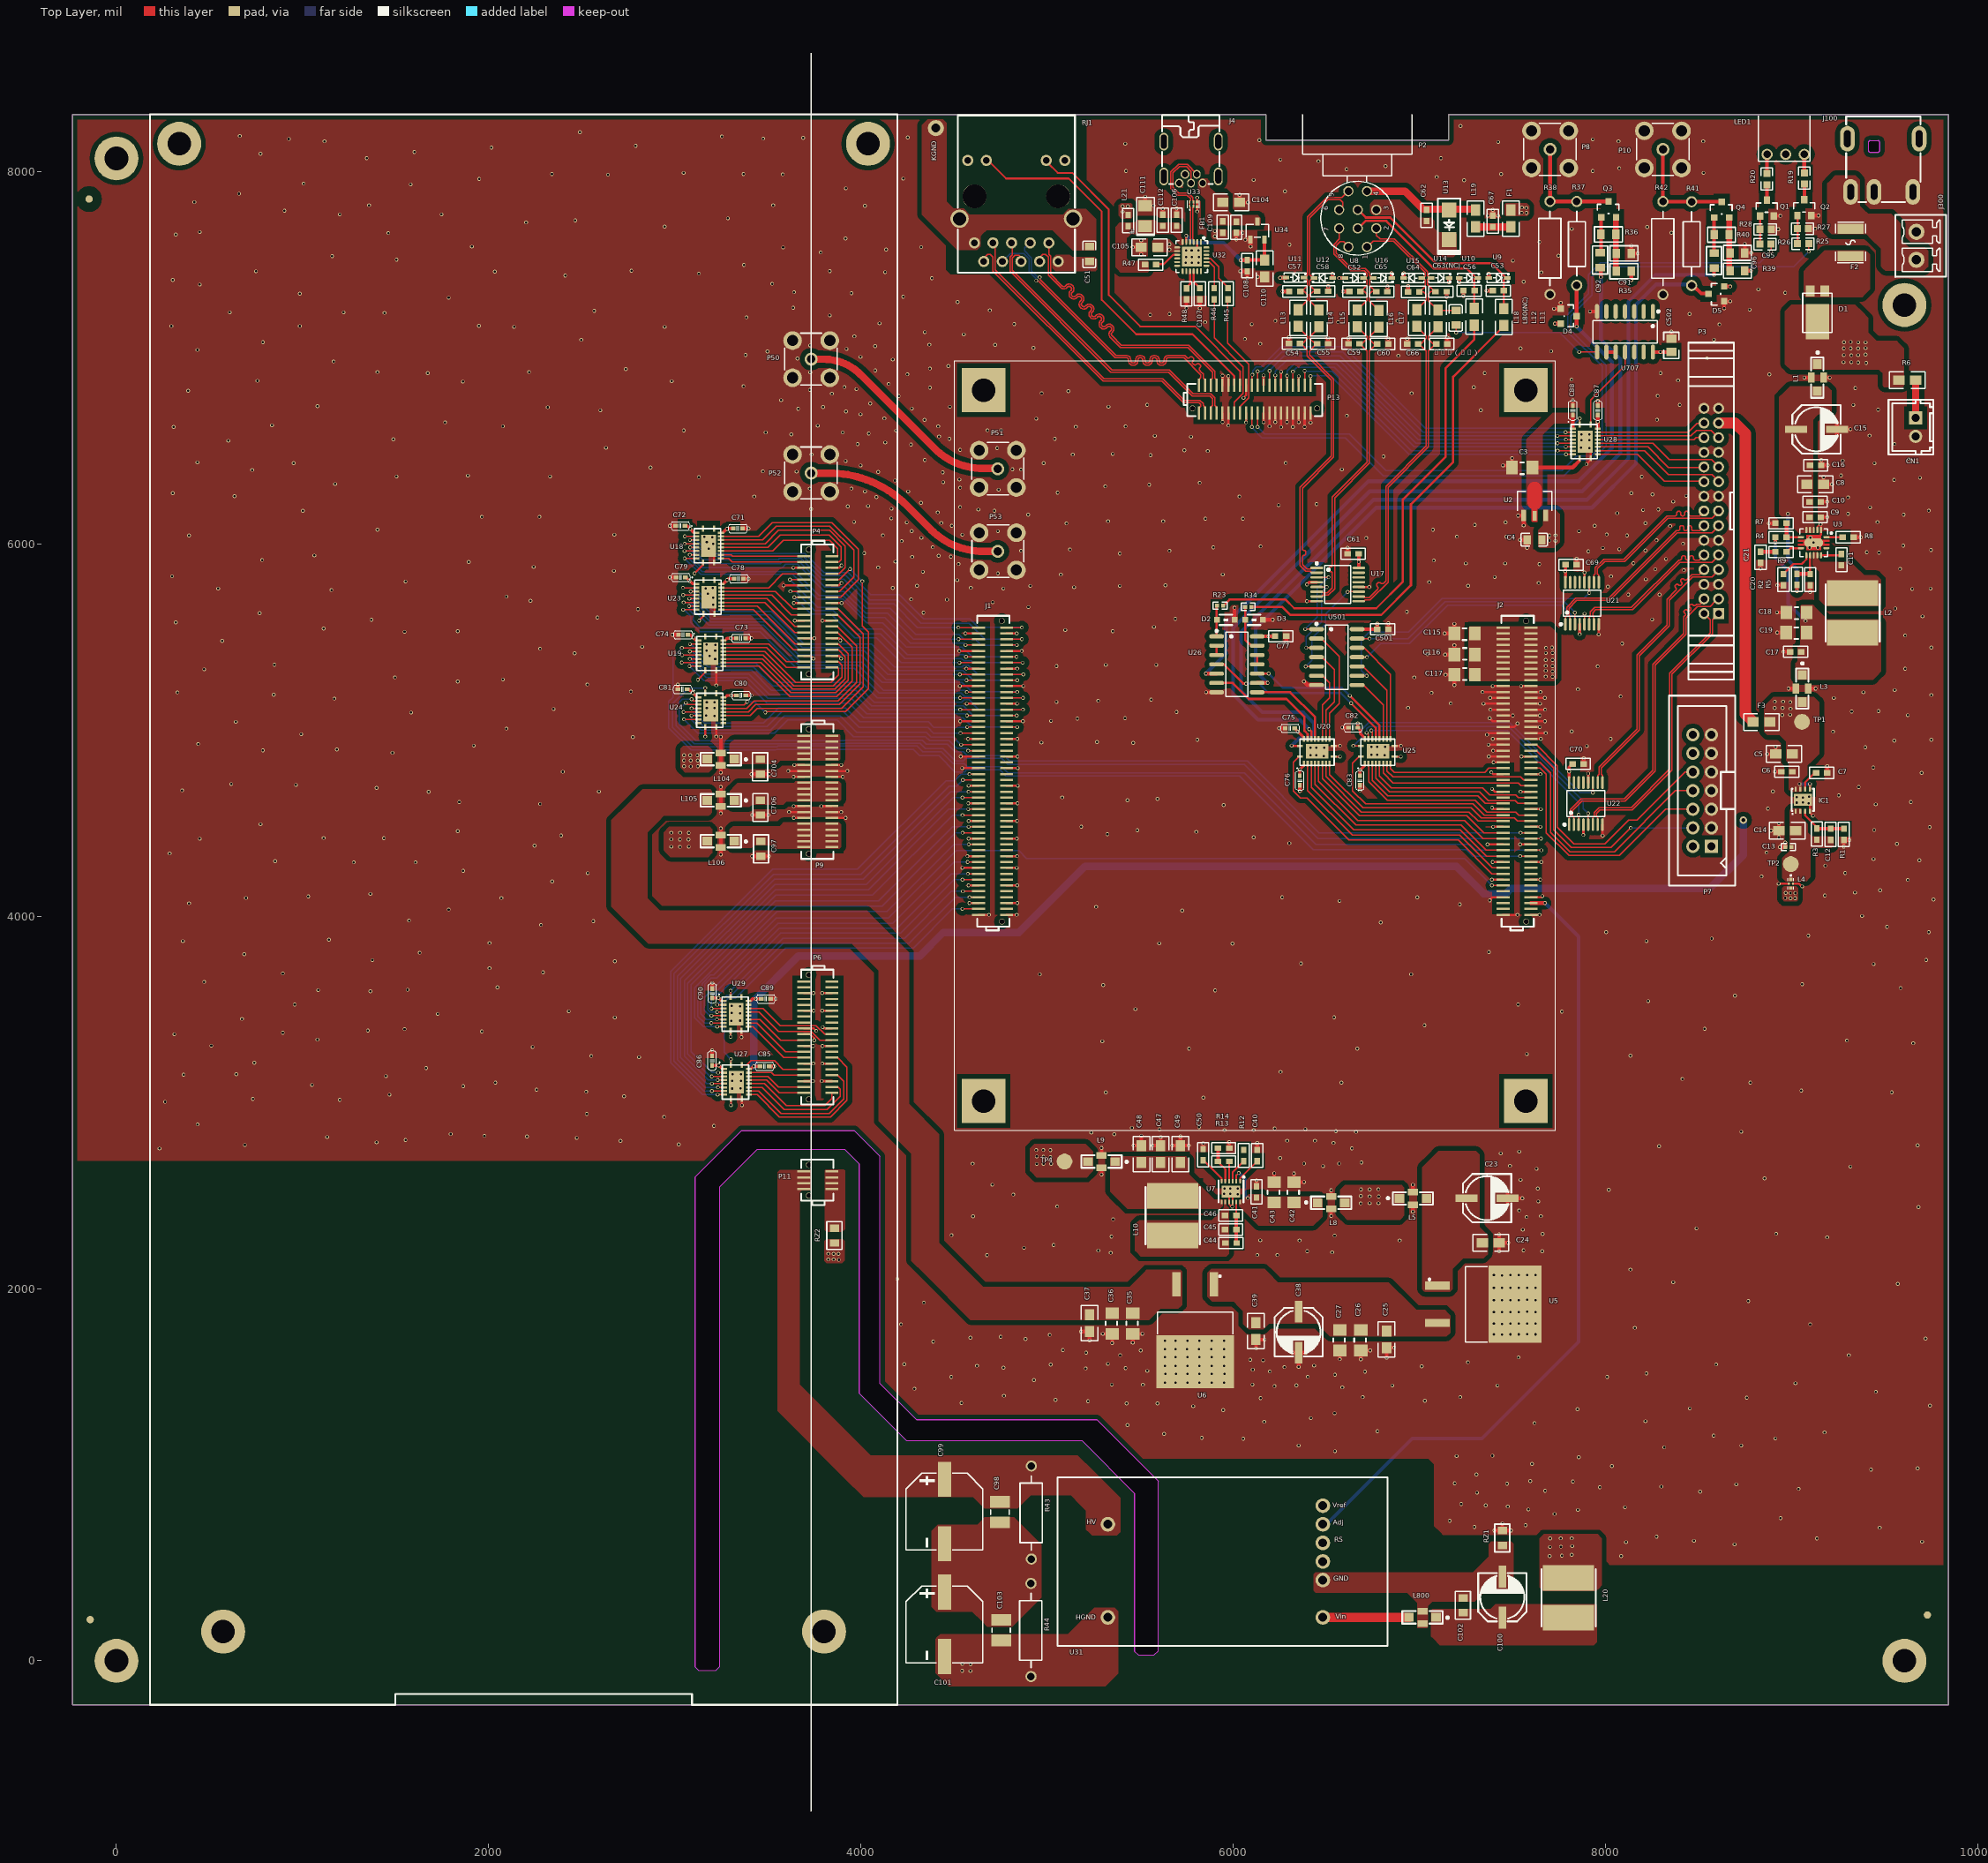
[diagram p0: Top Layer view]
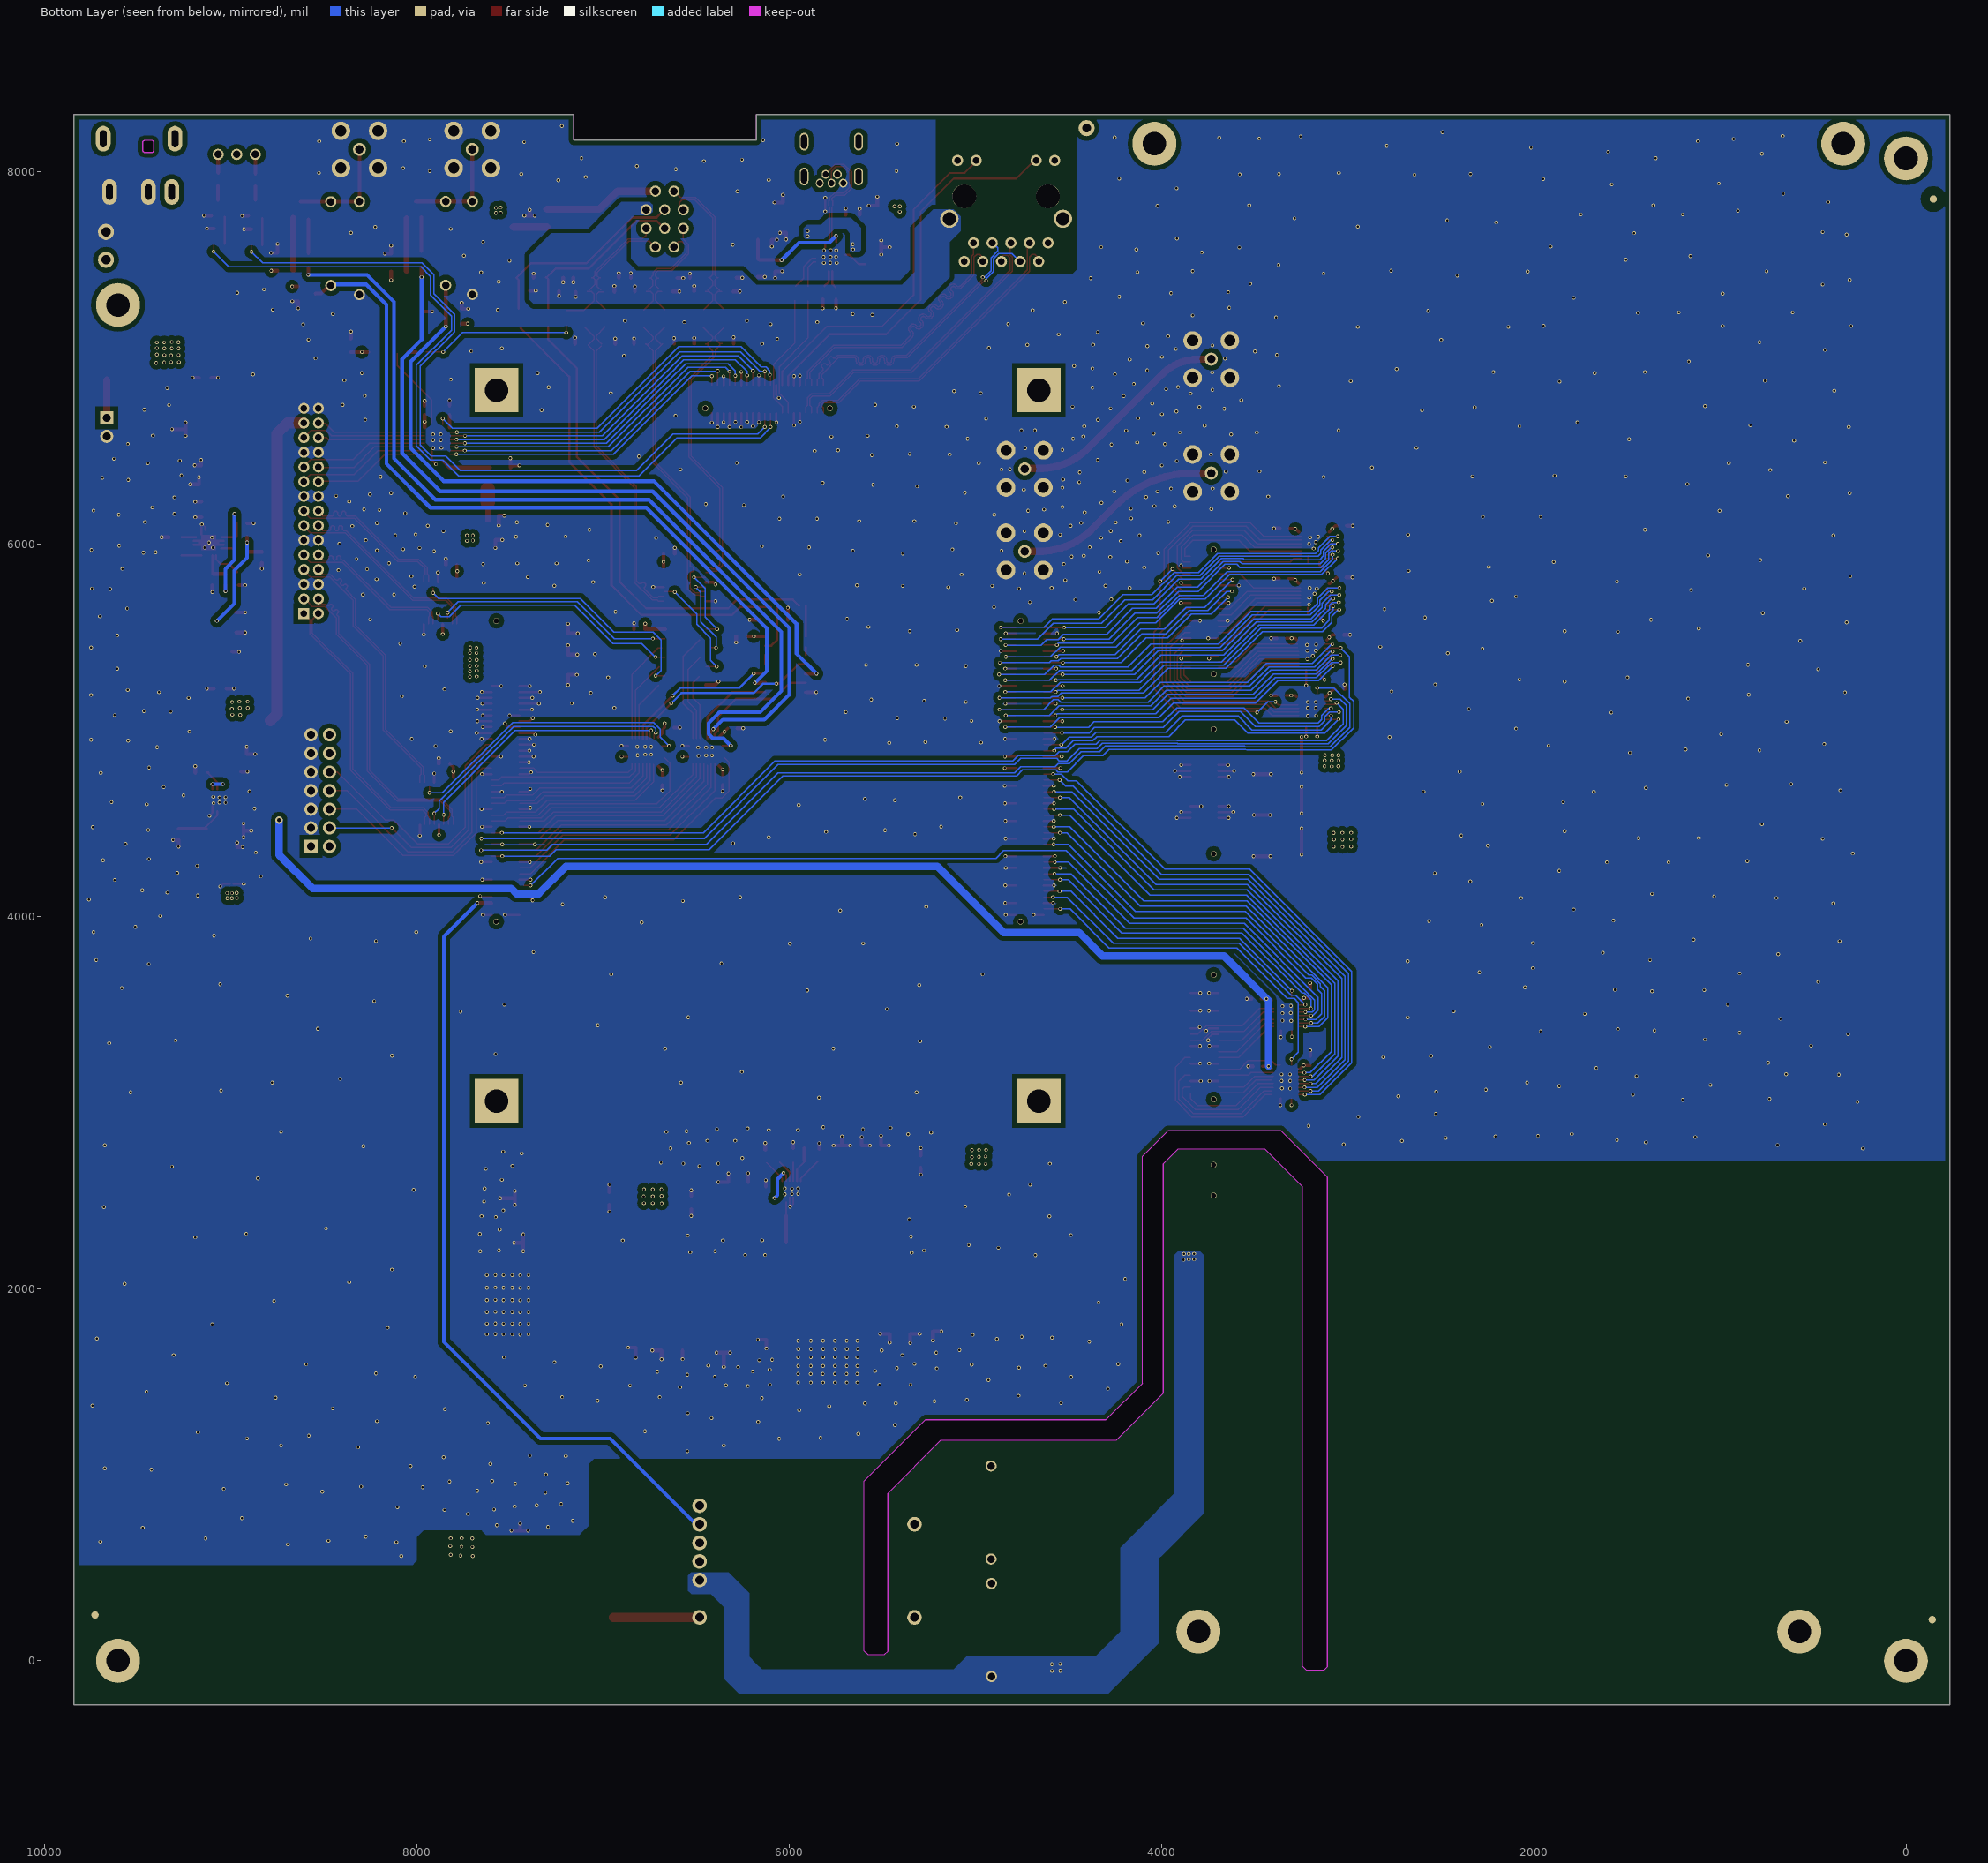
[diagram p1: Bottom Layer view, seen from below]
# Altium PCB MISC82191.PcbDoc (part 1 of 9)
Units mil, origin at the board's own origin, x right, y up, seen from the top; angles counter-clockwise.
Board outline 10078.74 x 8543.31 mil, 4 copper layers (Top Layer, GND, POWER, Bottom Layer); 238 components, 299 nets, 1297 pads, 1665 vias.

## Layer stack, top to bottom (the 12.6 mil dielectric is the usual default, probably not edited)
Top Layer: signal copper 1.4
Dielectric: core 12.6, FR-4, Dk 4.8
GND: plane copper 1.4, net GND
Dielectric: prepreg 12.6, FR-4, Dk 4.8
POWER: plane copper 1.4, net (Multiple Nets)
Dielectric: core 12.6, FR-4, Dk 4.8
Bottom Layer: signal copper 1.4

## Board outline
-236.22,-236.22 -236.22,8307.09 6175.79,8307.09 6175.79,8169.29 7157.25,8169.29 7157.25,8307.09 9842.52,8307.09 9842.52,-236.22
cut-out: 3128.78,-50.22 3220.78,-50.22 3240.78,-30.22 3240.78,2546.78 3442.78,2748.78 3911.78,2748.78 3990.78,2669.78 3990.78,1436.78 4244.78,1182.78 5187.78,1182.78 5470.78,899.78 5470.78,51.78 5490.78,31.78 5574.78,31.78 5596.78,53.78 5596.78,965.78 5267.78,1294.78 4297.78,1294.78 4102.78,1489.78 4102.78,2710.78 3965.78,2847.78 3357.78,2847.78 3109.78,2599.78 3109.78,-31.22

## Design rules (kind name [scope] priority, off if disabled: settings)
Clearance Clearance_2 [HASPAD('FREE-MARK')] p1: gap=50
Clearance Clearance_1 [INPOLYGON] p2: gap=6
Clearance [All] p3: gap=6
DiffPairsRouting [All] p1: maxlimit=6 minlimit=6 mostfreqgap=6 maxuncoupledlength=500
HoleSize [All] p1: absolutevalues=TRUE maxlimit=500 minlimit=1 maxpercent=80.000 minpercent=20.000
HoleToHoleClearance [All] p1: gap=0 allowstackedmicrovias=TRUE
MinimumSolderMaskSliver [All] p1: minsoldermaskwidth=0
PlaneClearance [All] p1: clearance=6
PlaneConnect [All] p1: planeconnectstyle=Direct reliefexpansion=20 reliefentries=4 reliefconductorwidth=10 reliefairgap=10
PolygonConnect [All] p1: connectstyle=Direct reliefconductorwidth=10 reliefentries=4 polygonreliefangle="90 Angle"
RoutingVias [All] p1: holewidth=12 width=20 viastyle="Through Hole" minholewidth=12 minwidth=20 maxholewidth=12 maxwidth=20
SilkToSilkClearance [All] p1: silktosilkclearance=0
SilkscreenOverComponentPads [IsPad] p1: minsilkscreentomaskgap=0
SolderMaskExpansion [All] p1: expansion=4
Width [All] p1: maxlimit=100 minlimit=6 preferedwidth=6 minimp=50.000000 maximp=50.000000 favimp=50.000000
20 further rules are at their usual default settings.

## Classes and differential pairs
component class FPGA_IO: C51 C52 C53 C54 C55 C56 C57 C58 C59 C60 C61 C62 C63(NC) C64 C65 C66 C67 C68（NC） C69 C70 C71 C72 C73 C74 C75 C76 C77 C78 C79 C80 C81 C82 C83 C85 C86 C87 C88 C89 C90 C91 C92 C95 C96 C97 C98 C99 C100 C101 C102 C103 C115 C116 C117 C501 C502 C704 C706 D2 D3 D4 D5 F1 F3 J1 J2 L11 L12 L13 L14 L15 L16 L17 L18 L19 L20 L80(NC) L104 L105 L106 L800 LED1 P2 P3 P4 P6 P7 P8 P9 P10 P11 P13 P50 P51 P52 P53 Q1 Q2 Q3 Q4 R19 R20 R23 R25 R26 R27 R28 R34 R35 R36 R37 R38 R39 R40 R41 R42 R43 R44 RJ1 RZ1 RZ2 U8 U9 U10 U11 U12 U13 U14 U15 U16 U17 U18 U19 U20 U21 U22 U23 U24 U25 U26 U27 U28 U29 U31 U501 U707
component class FPGA_串口: C104 C105 C106 C107 C108 C109 C110 C111 C112 FB1 J4 L21 R45 R46 R47 R48 U32 U33 U34
component class 电源: C3 C4 C5 C6 C7 C8 C9 C10 C11 C12 C13 C14 C15 C16 C17 C18 C19 C20 C21 C23 C24 C25 C26 C27 C29 C30 C35 C36 C37 C38 C39 C40 C41 C42 C43 C44 C45 C46 C47 C48 C49 C50 CN1 D1 F2 IC1 J100 J300 L1 L2 L3 L4 L5 L8 L9 L10 R1 R2 R3 R4 R5 R6 R7 R8 R9 R12 R13 R14 TP1 TP2 TP4 U2 U3 U5 U6 U7
differential pair D_ETH_TD3: +ETH_TD3_P -ETH_TD3_N
differential pair D_ETH_TD2: +ETH_TD2_P -ETH_TD2_N
differential pair D_ETH_TD1: +ETH_TD1_P -ETH_TD1_N
differential pair D_ETH_TD0: +ETH_TD0_P -ETH_TD0_N
differential pair "D_ENCODER Z": +"ENCODER Z_P" -"ENCODER Z_N"
differential pair "D_ENCODER B": +"ENCODER B_P" -"ENCODER B_N"
differential pair "D_ENCODER A": +"ENCODER A_P" -"ENCODER A_N"
differential pair "ENCODER A": +"ENCODER A_P" -"ENCODER A_N"
differential pair "ENCODER B": +"ENCODER B_P" -"ENCODER B_N"
differential pair "ENCODER Z": +"ENCODER Z_P" -"ENCODER Z_N"
differential pair ETH_TD0: +ETH_TD0_P -ETH_TD0_N
differential pair ETH_TD1: +ETH_TD1_P -ETH_TD1_N
differential pair ETH_TD2: +ETH_TD2_P -ETH_TD2_N
differential pair ETH_TD3: +ETH_TD3_P -ETH_TD3_N
differential pair NewDifferentialPair1: +USB_UART_D- -USB_UART_D+
differential pair D_2_A: +2_A_P -2_A_N
differential pair D_3_A: +3_A_P -3_A_N
differential pair D_1_A: +1_A_P -1_A_N
differential pair D_USB_UART_D: +USB_UART_D+ -USB_UART_D-
differential pair "D_ENCODER3 Z": +"ENCODER3 Z+" -"ENCODER3 Z-"
differential pair "D_ENCODER3 B": +"ENCODER3 B+" -"ENCODER3 B-"
differential pair "D_ENCODER3 A": +"ENCODER3 A+" -"ENCODER3 A-"
differential pair "D_ENCODER2 Z": +"ENCODER2 Z+" -"ENCODER2 Z-"
differential pair "D_ENCODER2 B": +"ENCODER2 B+" -"ENCODER2 B-"
differential pair "D_ENCODER2 A": +"ENCODER2 A+" -"ENCODER2 A-"

## Components (designator, comment, footprint, x,y, rotation, side; value= is the part's Value field where it differs from the comment)
C3 "22uf" 1206 7607.78,6410.16 r270 top
C4 "10uf" 0805A 7578.78,6021.16 r90 top
C5 "22uF/16V" 0805#1 8914.78,4871.16 r0 top
C6 "100nF" 0603#1 8974.78,4776.16 r90 top
C7 "100nF" 0603#1 9161.78,4770.16 r270 top
C8 "10uF 25V" 0805#1 9081.52,6320.09 r0 top
C9 "4.7uF 25V" 0603#1 9126.78,6143.16 r90 top
C10 "100nF 25V" 0603#1 9126.78,6226.16 r90 top
C11 "100nF 25V" 0603#1 9267.78,5915.16 r0 top
C12 "10nF" 0603#1 9209.78,4440.16 r0 top
C13 "100nF" 0402 8982.78,4372.16 r180 top
C14 "22uF/16V" 0805#1 8931.78,4459.16 r0 top
C15 "220UF 25V (D6.3*7.7mm)" CAP-SMD-6.3 9036.52,6613.09 r0 top
C16 "100NF 10%" 0603#1 9129.52,6422.09 r90 top
C17 "100nF 25V" 0603#1 9021.78,5420.16 r270 top
C18 "47uF 25V" 1206 9081.78,5632.16 r270 top
C19 "47uF 25V" 1206 9080.78,5524.16 r270 top
C20 "10nF 25V" 0603#1 8956.78,5808.16 r0 top
C21 "8200pF 25V" 0603#1 8833.03,5928.41 r0 top
C23 "220UF 25V (D6.3*7.7mm)" CAP-SMD-6.3 7266.73,2482.59 r0 top
C24 "330nF 10%" 0805#1 7428.73,2245.59 r180 top
C25 "100nF 10%" 0805#1 6824.4,1682.09 r90 top
C26 "47uF 25V" 1206 6685.59,1667.45 r180 top
C27 "47uF 25V" 1206 6572.59,1667.45 r180 top
C35 "47uF 25V" 1206 5460.59,1756.83 r180 top
C36 "47uF 25V" 1206 5349.59,1756.83 r180 top
C37 "100nF 10%" 0805#1 5227.59,1768.83 r90 top
C38 "220UF 25V (D6.3*7.7mm)" CAP-SMD-6.3 6348.59,1862.83 r270 top
C39 "330nF 10%" 0805#1 6122.59,1725.83 r90 top
C40 "220nF 25V" 0603#1 6128.59,2714.83 r0 top
C41 "2.2uF 25V" 0603#1 6125.59,2518.83 r180 top
C42 "22uF 25V" 1206 6326.59,2461.83 r180 top
C43 "22uF 25V" 1206 6220.59,2461.83 r180 top
C44 "10uF 16V" 0603#1 5988.59,2244.83 r90 top
C45 "10uF 16V" 0603#1 5986.59,2316.83 r90 top
C46 "10uF 16V" 0603#1 5986.59,2392.83 r90 top
C47 "22uF 16V" 0805#1 5610.59,2767.83 r270 top
C48 "22uF 16V" 0805#1 5506.59,2767.83 r270 top
C49 "22uF 16V" 0805#1 5716.59,2767.83 r270 top
C50 "1uF 25V" 0603#1 5838.78,2719.16 r180 top
C51 "100NF 10%" 0805A 5228.78,7517.16 r180 top
C52 "10pF/50V" 0603#1 6653.78,7356.16 r270 top
C53 "10pF/50V" 0603#1 7423.78,7360.16 r270 top
C54 "10pF/50V" 0603#1 6328.78,7076.16 r270 top
C55 "10pF/50V" 0603#1 6480.78,7075.16 r90 top
C56 "10pF/50V" 0603#1 7266.78,7360.16 r270 top
C57 "10pF/50V" 0603#1 6330.78,7356.16 r270 top
C58 "10pF/50V" 0603#1 6480.78,7357.16 r90 top
C59 "10pF/50V" 0603#1 6648.78,7075.16 r270 top
C60 "10pF/50V" 0603#1 6803.78,7074.16 r90 top
C61 "100nF/50V" 0603#1 6644.78,5947.16 r90 top
C62 "10pF/50V" 0603#1 7038.78,7764.23 r180 top
C63(NC) "10pF/50V" 0603#1 7116.78,7355.16 r270 top
C64 "10pF/50V" 0603#1 6969.78,7354.16 r90 top
C65 "10pF/50V" 0603#1 6798.78,7355.16 r270 top
C66 "10pF/50V" 0603#1 6964.78,7074.16 r270 top
C67 "10pF/50V" 0603#1 7394.78,7733.16 r0 top
C68（NC） "10pF/50V" 0603#1 7120.78,7074.16 r90 top
C69 "100nF/50V" 0603#1 7814.78,5888.16 r270 top
C70 "100nF/50V" 0603#1 7852.78,4818.16 r270 top
C71 "100NF" C0402 3313.78,6083.16 r0 top
C72 "100NF" C0402 3004.78,6097.16 r0 top
C73 "100NF" C0402 3330.78,5493.16 r0 top
C74 "100NF" C0402 3019.78,5512.16 r0 top
C75 "100NF" C0402 6329.78,5009.16 r180 top
C76 "100NF" C0402 6357.78,4704.16 r90 top
C77 "100NF" 0603#1 6254.78,5504.16 r270 top
C78 "100NF" C0402 3318.78,5813.16 r0 top
C79 "100NF" C0402 3006.78,5820.16 r0 top
C80 "100NF" C0402 3331.78,5186.16 r0 top
C81 "100NF" C0402 3016.78,5219.16 r0 top
C82 "100NF" C0402 6668.78,5013.16 r180 top
C83 "100NF" C0402 6680.78,4704.16 r90 top
C85 "100NF" C0402 3457.78,3194.16 r0 top
C86 "100NF" C0402 3200.78,3249.16 r270 top
C87 "100NF" C0402 7958.78,6692.16 r90 top
C88 "100NF" C0402 7824.78,6742.16 r270 top
C89 "100NF" C0402 3464.78,3556.16 r0 top
C90 "100NF" C0402 3201.78,3611.16 r270 top
C91 "100NF 10%" 0805R 8058.78,7560.16 r0 top
C92 "150PF 10%" 0805R 7971.78,7485.16 r90 top
C95 "100NF 10%" 0805R 8668.78,7563.16 r0 top
C96 "150PF 10%" 0805R 8583.78,7482.16 r90 top
C97 "10uF  25V 10%" 0805R 3462.78,4401.78 r270 top
C98 "1KV/1nF" 3225[1210] 4746.78,798.78 r270 top
C99 "500V 10UF" CAP-SMD_BD10.0-L10.3-W10.3-LS11.0-R-RD 4448.59,974.83 r90 top
C100 "220UF 25V (D6.3*7.7mm)" CAP-SMD-6.3 7448.78,244.78 r90 top
C101 "500V 10UF" CAP-SMD_BD10.0-L10.3-W10.3-LS11.0-R-RD 4448.59,368.83 r90 top
C102 "100NF 10%" 0805R 7234.78,258.41 r90 top
C103 "1KV/1nF" 3225[1210] 4753.52,165.09 r270 top
C104 "10uf" 0805#1 6033.78,7834.16 r180 top
C105 "10uf" 0805#1 5595.78,7594.16 r180 top
C106 "100nF" 0603#1 5695.78,7738.16 r0 top
C107 "4.7uF" 0603#1 5820.78,7344.16 r180 top
C108 "100nF" 0603#1 6075.78,7494.16 r180 top
C109 "2.2uf" 0603#1 6016.78,7701.16 r180 top
C110 "10uf" 0805#1 6168.78,7434.16 r90 top
C111 "4.7UF 10V type A" 1005 5526.78,7707.16 r180 top
C112 "0.1uF 10%" 0603#1 5621.78,7738.16 r180 top
C115 "47uF 25V" 1206 7298.21,5519.18 r270 top
C116 "47uF 25V" 1206 7188.21,5405.18 r90 top
C117 "47uF 25V" 1206 7188.21,5297.18 r90 top
C501 "100nF/50V" 0603#1 6803.78,5541.16 r270 top
C502 "100nF/50V" 0603#2 8354.78,7102.78 r0 top
C704 "10uF  25V 10%" 0805R 3458.78,4762.78 r90 top
C706 "10uF  25V 10%" 0805R 3459.78,4543.78 r90 top
CN1 "#NAME?" CONN-TH_2P-P2.50_HX25003-2A 9666.52,6627.09 r270 top
D1 "SB1045L" SB1045L 9138.52,7194.09 r270 top
D2 "BV08C" SOD323 5959.78,5592.16 r180 top
D3 "BV08C" SOD323 6111.78,5592.16 r180 top
D4 "BAV99/A7" SOT-23 7759.78,7263.16 r270 top
D5 "BAV99/A7" SOT-23 8637.78,7303.16 r90 top
F1 "Fuse  6V 0.2A" 0805#1 7490.78,7703.16 r90 top
F2 "16V 4A" 1812 9316.78,7692.41 r270 top
F3 "Fuse  6V 0.2A" 0805#1 8792.78,5043.78 r0 top
FB1 "100R" 0603#1 5943.78,7702.16 r0 top
IC1 "TPL910A" DFN-8_L3.0-W3.0-P0.65-BL-EP2.3 9021.78,4563.16 r0 top
J1 "0.8mm 2*50" 板对板座2*50 4782.37,5550.98 r90 top locked
J2 "0.8mm 2*50" 板对板座2*50 7599.01,5550.98 r90 top locked
J4 "Micro_USB2.0_DIP1" MINI-USB-TH_USB-MINI-2 5835.78,7938.16 r180 top
J100 "DC-044A-A250" DC-IN-TH_DC-044A-A250 9317.4,7891.09 r270 top
J300 "WJ15EDGVC-3.81-2P" CONN-TH_WJ15EDGVC-3.81-2P 9670.78,7526.41 r90 top
L1 "YFF31HC2A105MT000N" FILTER-SMD_4P-L3.2-W1.6-L_YFF31HC 9138.52,6966.09 r270 top
L2 "SLF0705-2R2MTT (2.2uH 6A)" IND-SMD_L7.8-W7.0-A 9327.78,5523.16 r90 top
L3 "YFF31HC2A105MT000N" FILTER-SMD_4P-L3.2-W1.6-L_YFF31HC 9056.78,5296.16 r270 top
L4 "YFF15PC0G435MT000N" FILTER-SMD_4P-L1.0-W0.5-L 8995.78,4197.16 r270 top
L5 "YFF31HC2A105MT000N" FILTER-SMD_4P-L3.2-W1.6-L_YFF31HC 6892.97,2483.73 r0 top
L8 "YFF31HC2A105MT000N" FILTER-SMD_4P-L3.2-W1.6-L_YFF31HC 6453.59,2460.83 r0 top
L9 "YFF31HC2A105MT000N" FILTER-SMD_4P-L3.2-W1.6-L_YFF31HC 5365.59,2681.83 r180 top
L10 "XRCD54-4R7M(4.7uH 2A SMD,4.5x5.2mm)" IND-SMD_L7.8-W7.0-A 5674.78,2498.16 r270 top
L11 "600Ω-1.3A" 0805#1 7453.78,7173.16 r90 top
L12 "600Ω-1.3A" 0805#1 7294.78,7175.16 r90 top
L13 "600Ω-1.3A" 0805#1 6349.78,7168.16 r90 top
L14 "600Ω-1.3A" 0805#1 6460.78,7166.16 r90 top
L15 "600Ω-1.3A" 0805#1 6667.78,7166.16 r90 top
L16 "600Ω-1.3A" 0805#1 6783.78,7164.16 r90 top
L17 "600Ω-1.3A" 0805#1 6985.78,7168.16 r90 top
L18 "600Ω-1.3A" 0805#1 7099.78,7166.16 r90 top
L19 "600Ω-1.3A" 0805#1 7302.78,7703.16 r90 top
L20 "XRCD54-4R7M(4.7uH 2A SMD,4.5x5.2mm)" IND-SMD_L7.8-W7.0-A 7801.78,444.78 r270 top
L21 "600Ω-1.3A" 0603#1 5435.78,7737.16 r180 top
L80(NC) "600Ω-1.3A" 0805#2 7197.4,7175.09 r180 top
L104 "YFF31HC2A105MT000N" FILTER-SMD_4P-L3.2-W1.6-L_YFF31HC 3319.78,4843.78 r180 top
L105 "YFF31HC2A105MT000N" FILTER-SMD_4P-L3.2-W1.6-L_YFF31HC 3319.78,4622.78 r180 top
L106 "YFF31HC2A105MT000N" FILTER-SMD_4P-L3.2-W1.6-L_YFF31HC 3319.78,4402.78 r180 top
L800 "YFF31HC2A105MT000N" FILTER-SMD_4P-L3.2-W1.6-L_YFF31HC 7089.78,233.41 r180 top
LED1 "LED white body, red/green bicolour(Φ3/common anode) with 3mm single-hole square LED right-angle holder(7*6.4*7.4mm)" DIP3B 8868.33,8092.36 r90 top
P2 "Header 10" 2B-10 6718.78,7595.16 r0 top
P3 "MTE220-30SL" CONN-TH_MTE220-30SL 8607.78,5625.78 r90 top locked
P4 "Header 20X2" N0.8mm/40Pin-Plug 3694.21,5934.26 r270 top
P6 "Header 20X2" N0.8mm/40Pin-Plug 3694.21,3649.78 r270 top
P7 "Header 7X2" IDC-TH_14P-P2.54-V-R2-C7-S2.54 8569.78,4374.78 r90 top
P8 "RF connector SMB-JWHD SMB right-angle male" DIP-P 7602.78,8019.16 r90 top
P9 "Header 20X2" N0.8mm/40Pin-Plug 3694.21,4969.15 r270 top
P10 "RF connector SMB-JWHD SMB right-angle male" DIP-P 8208.78,8019.16 r90 top
P11 "Header 4X2" N0.8mm/8Pin-SOCKET 3694.21,2534.37 r270 top locked
P13 "Header 20X2" N0.8mm/40Pin-Plug 5816.67,6702.82 r0 top locked
P50 "Analog output" DIP-P 3632.78,6892.41 r90 top
P51 "AD input" DIP-P 4634.78,6503.16 r0 top locked
P52 "gain" DIP-P 3632.78,6280.6 r90 top
P53 "" DIP-P 4635.17,6059.85 r0 top locked
Q1 "MMBT3904LT1(1AM)" SOT23 8830.33,7762.36 r0 top
Q2 "MMBT3904LT1(1AM)" SOT23 9031.33,7763.36 r0 top